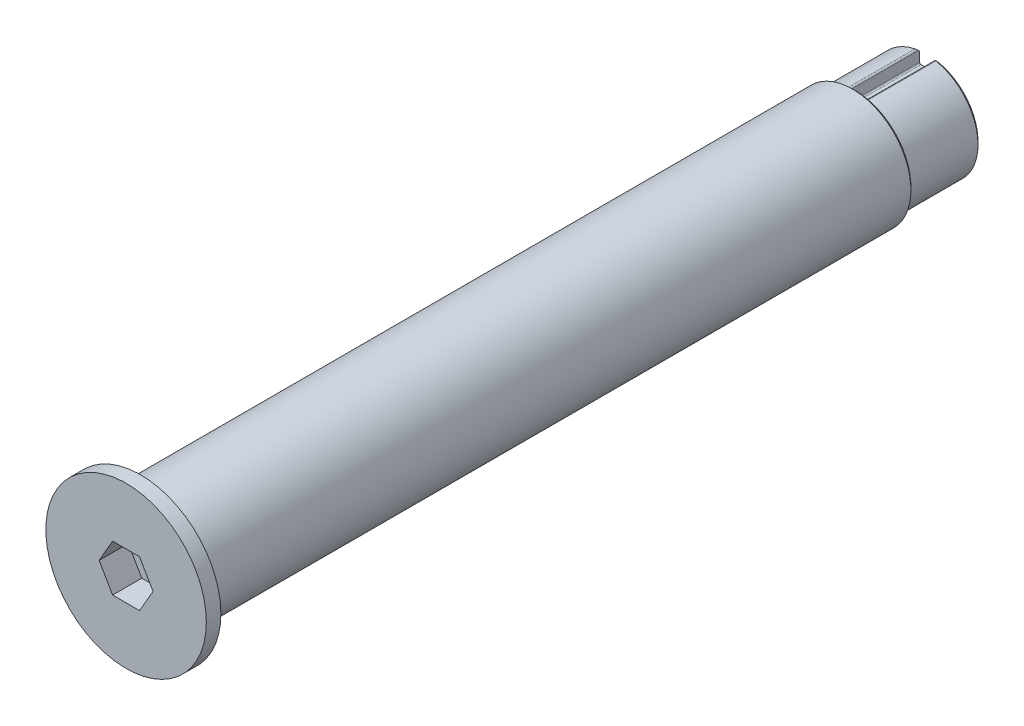
SolidWorks part; units mm, degrees
material "42CrMo"
ref_plane "前视基准面" through (0, 0, 0) normal (0, 0, 1) x (1, 0, 0)
ref_plane "上视基准面" through (0, 0, 0) normal (0, 1, 0) x (1, 0, 0)
ref_plane "右视基准面" through (0, 0, 0) normal (1, 0, 0) x (0, 0, -1)
sketch "草图1" plane through (0, 0, 0) normal (0, 0, 1) x (1, 0, 0)
  circle A0 centre (0, 0) radius 20
  dimension "D1" = 40
extrude "凸台-拉伸1" add sketch "草图1" along normal blind 270
sketch "草图2" plane through (0, 0, 270) normal (0, 0, 1) x (1, 0, 0)
  circle A0 centre (0, 0) radius 27.5
  dimension "D1" = 55
extrude "凸台-拉伸2" add sketch "草图2" along normal blind 5
sketch "草图3" plane through (0, 0, 275) normal (0, 0, 1) x (1, 0, 0)
  line L1 (9.2376, 0) -> (4.6188, 8)
  line L2 (4.6188, 8) -> (-4.6188, 8)
  line L3 (-4.6188, 8) -> (-9.2376, 0)
  line L4 (-9.2376, 0) -> (-4.6188, -8)
  line L5 (-4.6188, -8) -> (4.6188, -8)
  line L6 (4.6188, -8) -> (9.2376, 0)
  circle A0 centre (0, 0) radius 8 construction
  dimension "D1" = 16
extrude "切除-拉伸1" cut sketch "草图3" against normal blind 10
sketch "草图4" plane through (0, 0, 0) normal (0, 0, -1) x (-1, 0, 0)
  circle A0 centre (0, 0) radius 18
  dimension "D1" = 36
extrude "切除-拉伸2" cut sketch "草图4" against normal blind 25 flip side to cut
cosmetic thread "装饰螺纹线2" parameters "D2"=15
chamfer "倒角1" distance 1 angle 45 1 edges at (-20, 0, 25)
chamfer "倒角2" distance 1 angle 45 1 edges at (-18, 0, 0)
fillet "圆角1" radius 0.5 1 edges at (20, 0, 270)
sketch "草图5" plane through (0, 0, 0) normal (0, 0, -1) x (-1, 0, 0)
  line L0 (0, 0) -> (0, 18) construction
  line L1 (-3, 23) -> (3, 23)
  line L2 (-3, 23) -> (-3, 13)
  line L3 (-3, 13) -> (3, 13)
  line L4 (3, 23) -> (3, 13)
  line L5 (-3, 23) -> (3, 13) construction
  line L6 (-3, 13) -> (3, 23) construction
  circle A0 centre (0, 0) radius 18 construction
  circle A1 centre (0, 0) radius 18 construction
  point P0 (0, 18)
  dimension "D1" = 6
  dimension "D2" = 5
extrude "切除-拉伸3" cut sketch "草图5" against normal up to surface (25 mm away) up to face at (-19, 0, 25)
fillet "圆角2" radius 0.5 4 edges at (3, 13, 12.5) (-3, 13, 12.5) (-3, 17.7482, 13) (3, 17.7482, 13)
